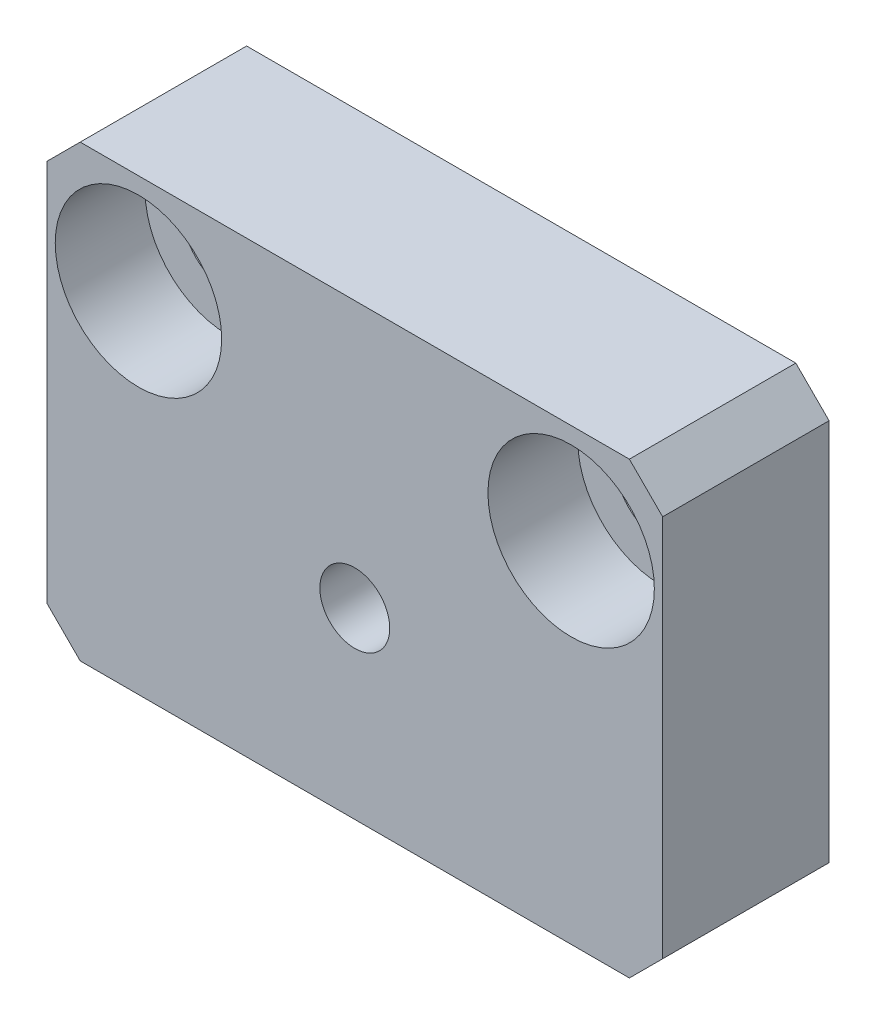
SolidWorks part; units mm, degrees
material "SS41"
ref_plane "Front Plane" through (0, 0, 0) normal (0, 0, 1) x (1, 0, 0)
ref_plane "Top Plane" through (0, 0, 0) normal (0, 1, 0) x (1, 0, 0)
ref_plane "Right Plane" through (0, 0, 0) normal (1, 0, 0) x (0, 0, -1)
sketch "Sketch1" plane through (0, 0, 0) normal (0, 0, 1) x (1, 0, 0)
  line L1 (-18.5, 13.5) -> (18.5, 13.5)
  line L2 (-18.5, 13.5) -> (-18.5, -13.5)
  line L3 (-18.5, -13.5) -> (18.5, -13.5)
  line L4 (18.5, 13.5) -> (18.5, -13.5)
  line L5 (-18.5, 13.5) -> (18.5, -13.5) construction
  line L6 (-18.5, -13.5) -> (18.5, 13.5) construction
  point P0 (0, 0)
  dimension "D1" = 37
  dimension "D2" = 27
extrude "Boss-Extrude1" add sketch "Sketch1" along normal blind 10
hole_wizard "CBORE for M5 Hex Socket Head Cap Screw1" positions "Sketch3" profile "Sketch2" counterbore size "M5" standard "Iso" end condition through all
sketch "Sketch3" plane through (0, 0, 10) normal (0, 0, 1) x (1, 0, 0)
  line L0 (0, 13.5) -> (0, 0) construction
  line L1 (18.5, 13.5) -> (-18.5, 13.5) construction
  point P0 (-13, 7.5)
  point P2 (13, 7.5)
  dimension "D1" = 6
  dimension "D2" = 26
sketch "Sketch2" plane through (-13, 7.5, 10) normal (1, 0, 0) x (0, -1, 0)
  line L0 (0, 0) -> (0, 10)
  line L1 (0, 10) -> (2.75, 10)
  line L3 (2.75, 10) -> (2.75, 5.4)
  line L4 (2.75, 5.4) -> (5, 5.4)
  line L5 (5, 5.4) -> (5, 0)
  line L7 (5, 0) -> (0, 0)
  line L11 (0, -6.35) -> (0, 107.95) construction
  dimension "通孔孔直径" = 5.5
  dimension "通孔孔深度" = 10
  dimension "柱形沉头孔直径" = 10
  dimension "柱形沉头孔深度" = 5.4
hole_wizard "M5 Tapped Hole1" positions "Sketch5" profile "Sketch4" tap size "M5" standard "Iso"
sketch "Sketch5" plane through (0, 0, 10) normal (0, 0, 1) x (1, 0, 0)
  line L0 (0, 13.5) -> (0, 0) construction
  line L1 (18.5, 13.5) -> (-18.5, 13.5) construction
  line L3 (-18.5, -13.5) -> (18.5, -13.5) construction
  point P0 (0, -2.5)
  dimension "D1" = 11
sketch "Sketch4" plane through (0, -2.5, 10) normal (1, 0, 0) x (0, -1, 0)
  line L0 (0, 0) -> (0, 13.6618)
  line L1 (0, 13.6618) -> (2.1, 12.4)
  line L2 (2.1, 12.4) -> (2.1, 0)
  line L5 (2.1, 0) -> (0, 0)
  line L10 (0, 13.6618) -> (-2.1, 12.4) construction
  line L11 (0, -6.35) -> (0, 107.95) construction
  dimension "螺纹孔钻头直径" = 4.2
  dimension "螺纹孔钻头深度" = 12.4
  dimension "导头角度" = 118
cosmetic thread "Hole thread1"
chamfer "Chamfer1" distance 2 angle 45 4 edges at (-18.5, -13.5, 5) (18.5, -13.5, 5) (18.5, 13.5, 5) (-18.5, 13.5, 5)
